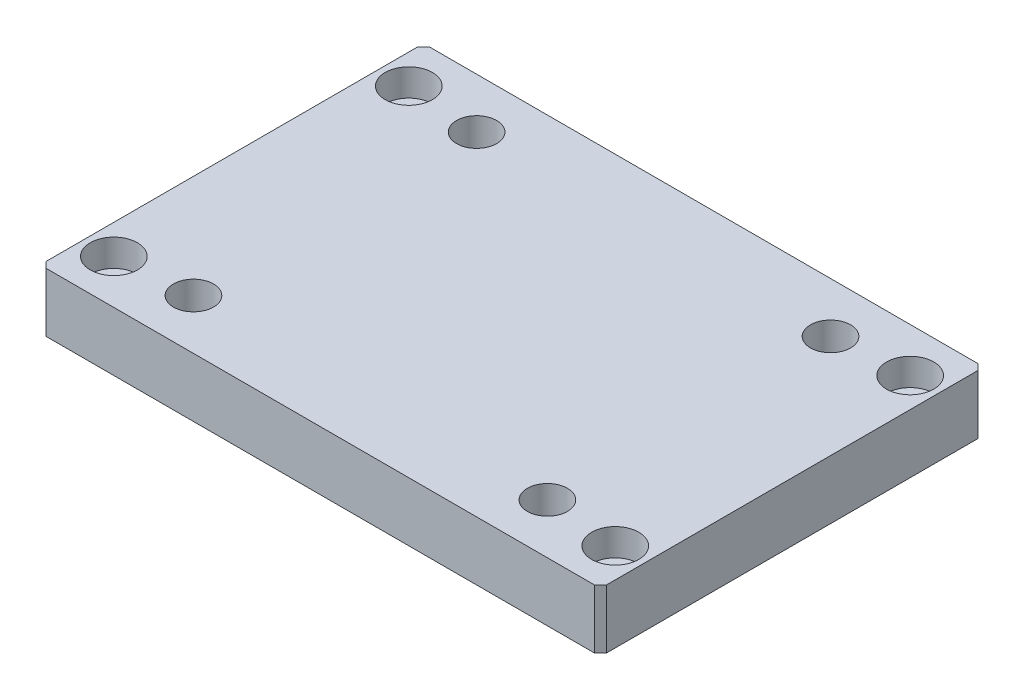
from build123d import *

# Parameters (mm, degrees)
SKETCH_1_W                   = 95
SKETCH_1_H                   = 65
EXTRUDE_1_DEPTH              = 5
CHAMFER_1_SIZE               = 1
HOLE_WIZARD_M4_1_D           = 4.5
HOLE_WIZARD_M4_1_CBORE_D     = 8
HOLE_WIZARD_M4_1_CBORE_DEPTH = 4.6
HOLE_WIZARD_M8_1_D           = 6.8


with BuildPart() as part:
    # 草图1 → 凸台-拉伸1 (new, symmetric)
    with BuildSketch(Plane(origin=(0, 0, 0), x_dir=(1, 0, 0), z_dir=(0, 1, 0))):
        Rectangle(SKETCH_1_W, SKETCH_1_H)
    extrude(amount=EXTRUDE_1_DEPTH, both=True)

    # 倒角1
    chamfer_1_edges = [part.edges().sort_by_distance(p)[0] for p in [
        (47.5, 0, 32.5),
        (-47.5, 0, 32.5),
        (-47.5, 0, -32.5),
        (47.5, 0, -32.5),
    ]]
    chamfer(chamfer_1_edges, length=CHAMFER_1_SIZE)

    # M4 六角圆柱头螺钉的柱形沉头孔1 (through all)
    with Locations(Plane(origin=(0, 5, 0), x_dir=(1, 0, 0), z_dir=(0, 1, 0))):
        with Locations((-42.5, 25), (-42.5, -25), (42.5, -25), (42.5, 25)):
            CounterBoreHole(HOLE_WIZARD_M4_1_D / 2, HOLE_WIZARD_M4_1_CBORE_D / 2, HOLE_WIZARD_M4_1_CBORE_DEPTH)

    # M8 螺纹孔1 (through all)
    with Locations(Plane(origin=(0, 5, 0), x_dir=(1, 0, 0), z_dir=(0, 1, 0))):
        with Locations((30, 24), (30, -24), (-30, -24), (-30, 24)):
            Hole(HOLE_WIZARD_M8_1_D / 2)


solid = part.part
